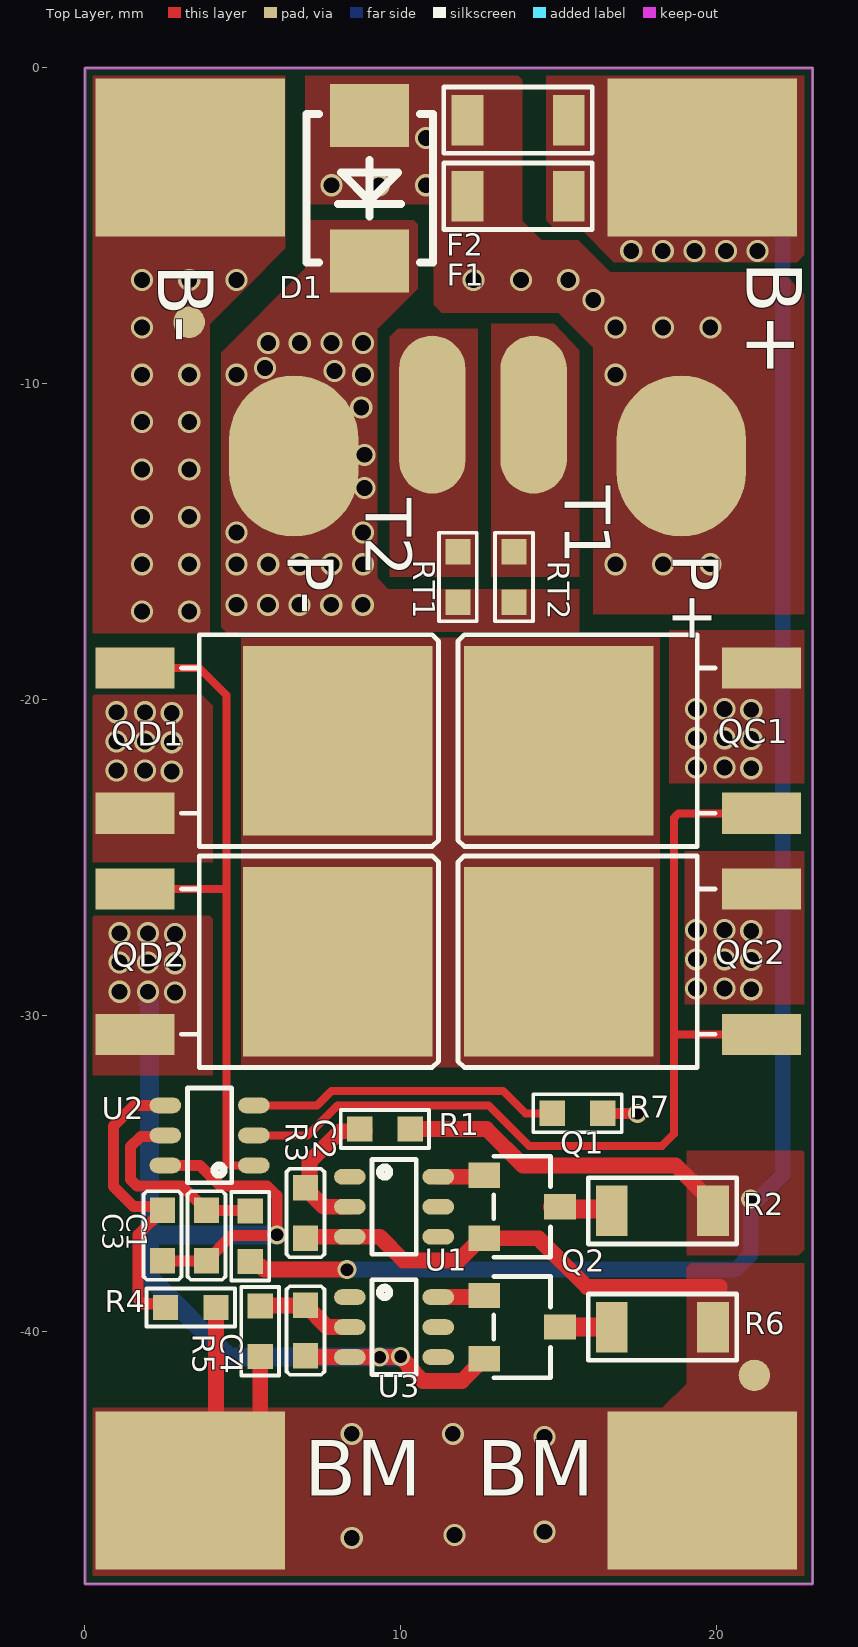
[diagram p0: Top Layer view]
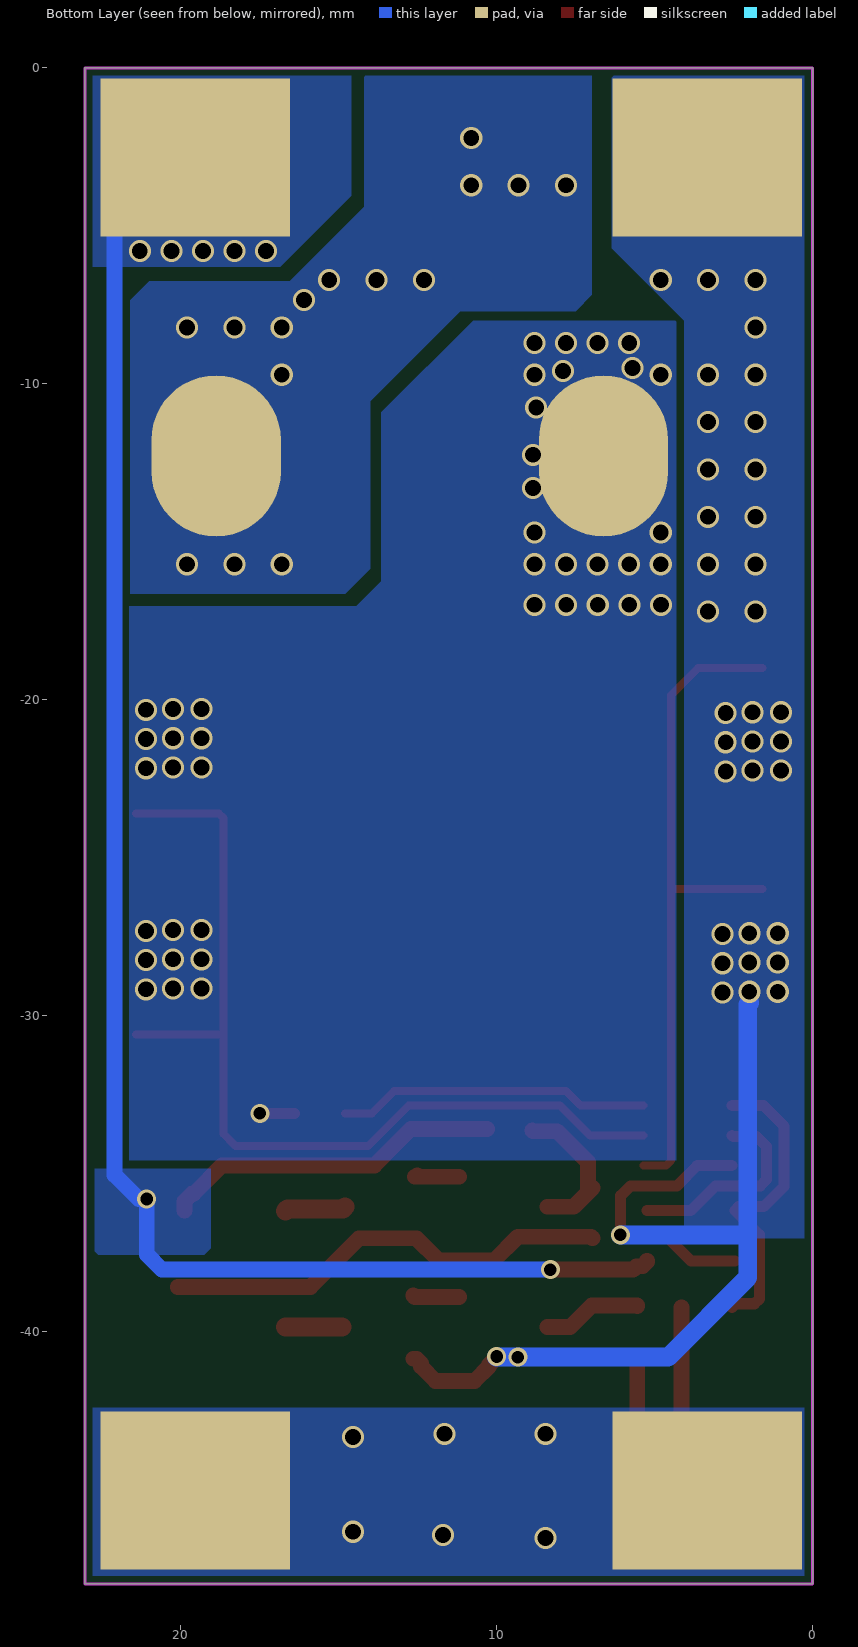
[diagram p1: Bottom Layer view, seen from below]
# Altium PCB MISC82045.PcbDoc
Units mm, origin at the board's own origin, x right, y up, seen from the top; angles counter-clockwise.
Board outline 23.04 x 48 mm, 2 copper layers (Top Layer, Bottom Layer); 33 components, 19 nets, 84 pads, 107 vias.

## Layer stack, top to bottom (the 12.6 mil dielectric is the usual default, probably not edited)
Top Solder: solder mask 0.0102, Solder Resist, Dk 3.5
Top Layer: signal copper 0.0356
Dielectric 1: dielectric 0.32, FR-4, Dk 4.8
Bottom Layer: signal copper 0.0356
Bottom Solder: solder mask 0.0102, Solder Resist, Dk 3.5

## Board outline
0,-48 23.039,-48 23.039,0 0,0

## Design rules (kind name [scope] priority, off if disabled: settings)
Clearance [All] p1: gap=0.2 ignorepadtopadclearanceinfootprint=FALSE
PolygonConnect [All] p1: connectstyle=Direct reliefconductorwidth=0.254 reliefentries=4 polygonreliefangle="90 Angle" airgapwidth=0.254
RoutingVias [All] p1: holewidth=0.711 width=1.27 viastyle="Through Hole" minholewidth=0.711 minwidth=1.27 maxholewidth=0.711 maxwidth=1.27
SilkToSilkClearance [All] p1: silktosilkclearance=0
SilkToSolderMaskClearance [IsPad] p1: minsilkscreentomaskgap=0 clearancetoexposedcopper=TRUE
SolderMaskExpansion [All] p1: expansion=0.102 istentingtop=FALSE
SupplyNets "Schematic Supply Nets" [InNet('P-')] p1: voltage=0.000
Width [All] p1: maxlimit=100 minlimit=0.254 preferedwidth=0.254
28 further rules are at their usual default settings.

## Components (designator, comment, footprint, x,y, rotation, side; value= is the part's Value field where it differs from the comment)
B+ "Pad" Pad10X8mm#1 19.546,-2.84 r90 top locked
B- "Pad" Pad10X8mm#2 4.156,-3.902 r90 top locked
BM "Pad" Pad10X8mm#1 19.546,-45.04 r90 top
BM "Pad" Pad10X8mm#1 3.338,-45.04 r270 top
C1 "0.1uF" C0603A 3.85,-36.971 r90 top
C2 "0.1uF" C0603A 6.983,-36.259 r90 top
C3 "0.1uF" C0603A 2.46,-36.971 r90 top
C4 "0.1uF" C0603A 6.985,-39.978 r90 top
D1 "RS2M" "SMB A (1+2-)" 9.017,-3.81 r90 top
F1 "F12F10 32V10A" R1206A 13.716,-4.064 r180 top
F2 "F12F10 32V10A" R1206A 13.716,-1.651 r180 top
P+ "Pad" Pad10X8mm#3 18.883,-12.286 r0 top
P- "Pad" Pad10X8mm#3 6.618,-12.286 r180 top
Q1 "3400" SOT23-3L 13.843,-36.06 r270 top
Q2 "3400" SOT23-3L 13.843,-39.87 r270 top
QC1 "N MOS*" TO-252 18.213,-21.3 r90 top
QC2 "N MOS*" TO-252 18.213,-28.3 r90 top
QD1 "N MOS*" TO-252 4.8,-21.3 r270 top
QD2 "N MOS*" TO-252 4.8,-28.3 r270 top
R1 "1K" R0603A 9.5,-33.6 r0 top
R2 "100R" R1206A 18.288,-36.187 r0 top
R3 "470R" R0603A 5.237,-36.996 r90 top
R4 "470R" R0603A 3.35,-39.25 r180 top
R5 "1K" R0603A 5.55,-40 r270 top
R6 "100R" R1206A 18.288,-39.87 r0 top
R7 "2K" R0603A 15.6,-33.1 r180 top
RT1 "NC" R0603A 11.811,-16.118 r90 top
RT2 "NC" R0603A 13.589,-16.118 r90 top
T1 "Pad" Pad10X8mm#4 14.208,-10.977 r180 top
T2 "Pad" Pad10X8mm#4 10.998,-10.977 r180 top
U1 "CM1010" SOT23-6A 9.79,-36.06 r0 top
U2 "S-8252*" SOT23-6A 3.95,-33.8 r180 top
U3 "CM1010" SOT23-6A 9.79,-39.87 r0 top

## Footprints (in the part's own frame and the unit in brackets; to place one, negate y for a bottom-side part, rotate by r counter-clockwise, add the part's x,y. Pads: shape width x height; smd on the part's side, far side on the other; paste and mask are expansions set on the pad)
C0603A [mm] "贴片电容"
  rect 0.8x0.8 smd mask+0.08: 1(-0.8,0) 2(0.8,0)
  silkscreen extent -1.4,-0.6 1.4,0.6
Pad10X8mm#1 [mm]
  rect 5x6 smd: 1(0,0)
Pad10X8mm#2 [mm]
  rect 5x6 smd: 1(1.062,0.818)
Pad10X8mm#3 [mm]
  oval 4.1x5.1 smd: 1(0,0)
Pad10X8mm#4 [mm]
  oval 2.1x5 smd: 1(0,0)
R0603A [mm] "贴片电阻"
  rect 0.8x0.8 smd mask+0.08: 1(-0.8,0) 2(0.8,0)
  silkscreen extent -1.4,-0.6 1.4,0.6
R1206A [mm] "贴片电阻"
  rect 1x1.6 smd: 1(-1.6,0) 2(1.6,0)
  silkscreen extent -2.35,-1.05 2.35,1.05
"SMB A (1+2-)" [mm] "贴片二极管"
  rect 2x2.5 smd: 1(2.3,0) 2(-2.3,0)
  silkscreen extent -2.35,-2 2.35,2
SOT23-3L [mm] "贴片IMOS"
  rect 0.8x1 smd: 1(-1,-1.2) 2(1,-1.2) 3(0,1.2)
  silkscreen extent -1.6,-0.9 1.6,0.9
SOT23-6A [mm]
  oval 1x0.5 smd mask+0.05: 1(-1.4,0.95) 2(-1.4,0) 3(-1.4,-0.95) 4(1.4,-0.95) 5(1.4,0) 6(1.4,0.95)
  silkscreen extent -0.7,-1.5 0.7,1.5
TO-252 [mm]
  rect 1.3x2.5 smd: 1(-2.3,-3.212) 2(2.3,-3.212)
  rect 6x6 smd: 3(0,3.213)
  silkscreen extent -3.35,-1.75 3.35,6.4

## Part data
B+ B- BM BM P+ P- T1 T2: "Connection pad (non-through-hole)"
C1 C2 C3 C4: library part CAP, "SMD capacitor"
D1: "SMD diode"
F1 F2: library part FUSE
Q1 Q2: library part "N MOS*", "SMD MOSFET"
QC1 QC2 QD1 QD2: "SMD MOSFET"
R1 R2 R3 R4 R5 R6 R7 RT1 RT2: library part RES, "SMD resistor"
U1 U3: "Chuangxinwei, balancing IC"
U2: library part S-8252, "2S battery protection IC"

## Free pads (board coordinates)
  rect 6x5 smd far side: 620(3.338,-45.04) 620(3.338,-2.84) 620(19.546,-45.04) 620(19.546,-2.84)
  oval 4.1x5.1 smd far side: 621(6.618,-12.286) 621(18.883,-12.286)
  round 1 smd: 622(3.3,-8.05) 622(21.2,-41.4)

## Via types
v1: diameter 0.7, hole 0.5, Top Layer to Bottom Layer, tented both sides, 101 vias
v2: diameter 0.6, hole 0.4, Top Layer to Bottom Layer, tented both sides, 6 vias

## Nets (pads, with @x,y where several pads share a name; then routed paths per layer and width w, separated by ;. In a path a pad name is that pad's centre, name@x,y a point inside that pad or via, vN(x,y) a via of type N, cw(c..) or ccw(c..) an arc to the next point about the centre after c; other vN are vias at no path point)
B+: B+.1 F1.1 F2.1 pad.620@19.546,-2.84 R1.2 R2.2 R3.1 | length 63.5
  Top Layer w0.5: R3.1@5.239,-37.771 5.239,-37.798 5.387,-37.946 5.576,-37.946 5.68,-38.05 v2(8.3,-38.05) ; R1.2 12.719,-33.6 13.869,-34.75 18.7,-34.75 19.587,-35.637 19.638,-35.637 19.888,-35.887 R2.2
  Bottom Layer w0.5: v2(8.3,-38.05) 20.6,-38.05 21.082,-37.568 v2(21.082,-35.814) 21.336,-35.814 22.1,-35.05 22.1,-5.09 19.85,-2.84 pad.620@19.546,-2.84
  other v1: 17.3,-5.8 18.3,-5.8 19.3,-5.8 20.3,-5.8 21.3,-5.8
B-: B-.1 C1.1 C3.1 C4.1 pad.620@3.338,-2.84 pad.622@3.3,-8.05 Q2.2 QD1.2 QD2.2 U2.6 U3.3 | length 37.4
  Top Layer w0.35: C3.1 C1.1 4.65,-36.971 6.135,-36.971 v2@6.198,-36.908 ; U2.6 3.65,-34.75 4.296,-35.396 5.767,-35.396 6.083,-35.712 v2(6.083,-36.95)
  Top Layer w0.5: C4.1 7.027,-40.82 U3.3 v2(9.332,-40.82) v2@10.02,-40.82 ; v2@10.019,-40.821 10.019,-40.846 10.24,-41.067 10.24,-41.11 10.704,-41.574 11.939,-41.574 12.393,-41.12 12.393,-41.02 12.543,-40.87 Q2.2
  Bottom Layer w0.6: v1@2,-29.6 2.05,-29.65 2.05,-36.95 ; v2(6.083,-36.95) 2.05,-36.95 ; v2@10,-40.82 4.57,-40.82 2.05,-38.3 2.05,-36.95
  other v1: 2.85,-29.275 1.1,-29.25 2,-29.25 2.85,-28.35 1.1,-28.325 2,-28.325 2.85,-27.425 1.1,-27.4 2,-27.4 2.75,-22.275 1,-22.25 1.9,-22.25 2.75,-21.35 1,-21.325 1.9,-21.325 2.75,-20.425 1,-20.4 1.9,-20.4 1.805,-17.214 3.305,-17.214 1.805,-15.714 3.305,-15.714 1.805,-14.214 3.305,-14.214 1.805,-12.714 3.305,-12.714 1.805,-11.214 3.305,-11.214 1.805,-9.714 3.305,-9.714 1.805,-8.214 1.805,-6.714 3.305,-6.714 4.805,-6.714
  other v2: 10,-40.8
BM: BM.1 C2.1 pad.620@3.338,-45.04 pad.620@19.546,-45.04 pad.622@21.2,-41.4 Q1.2 R4.1 R5.2 R6.2 U1.3 | length 27.4
  Top Layer w0.35: BM.1@1.443,-43.145 BM.1@3.338,-45.04
  Top Layer w0.5: BM.1@3.338,-45.04 BM.1@5.55,-42.828 ; BM.1@4.15,-44.328 R4.1 ; BM.1@5.55,-42.928 R5.2 ; C2.1@6.963,-37.059 7.012,-37.01 U1.3 9.332,-37.01 10.086,-37.764 11.839,-37.764 12.543,-37.06 Q1.2 14.36,-37.06 15.9,-38.6 20.1,-38.6
  other v1: 8.45,-46.55 11.7,-46.45 14.55,-46.35 14.55,-43.35 8.45,-43.25 11.65,-43.25
CO: QC1.1 QC2.1 U2.2 | length 30
  Top Layer w0.254: U2.2 7.05,-33.8 8,-32.85 12.785,-32.85 14.068,-34.132 18.268,-34.132 18.65,-33.75 18.65,-30.6 ; QC2.1 18.65,-30.6 ; QC1.1 18.799,-23.6 18.65,-23.749 18.65,-30.6
DO: QD1.1 QD2.1 U2.1 | length 21.8
  Top Layer w0.254: QD2.1 4.483,-26 ; QD1.1 3.62,-19 4.483,-19.864 4.483,-26 ; U2.1 4.632,-34.75 4.483,-34.601 4.483,-26
NetC1_2: C1.2 R3.2 U2.5 | length 6.5
  Top Layer w0.35: U2.5 2.521,-33.829 1.771,-33.829 1.45,-34.15 1.45,-35.191 1.655,-35.396 3.075,-35.396 C1.2 R3.2@5.239,-36.171
NetC2_2: C2.2 R1.1 U1.2 | length 4.7
  Top Layer w0.5: C2.2@6.963,-35.459 7.564,-36.06 U1.2 ; C2.2@7.113,-35.459 7.113,-34.637 8.08,-33.67 8.852,-33.67 R1.1@8.875,-33.647
NetC3_2: C3.2 R4.2 U2.4 | length 9.8
  Top Layer w0.35: R4.2 2.43,-39.13 1.83,-39.13 1.685,-38.985 1.685,-36.946 C3.2 2.343,-36.054 1.535,-36.054 0.9,-35.419 0.9,-33.505 1.555,-32.85 U2.4
NetC4_2: C4.2 R5.1 U3.2 | length 3.1
  Top Layer w0.5: R5.1 5.561,-39.189 6.974,-39.189 C4.2 7.677,-39.87 U3.2
NetQ1_1: Q1.1 U1.6 | length 1.5
  Top Layer w0.5: U1.6 Q1.1@12.593,-35.11 ; Q1.1@12.466,-35.11 Q1.1@12.516,-35.06
NetQ1_3: Q1.3 R2.1 | length 1.9
  Top Layer w0.6: Q1.3@14.8,-36.06 14.864,-36.123 16.625,-36.123 R2.1
NetQ2_1: Q2.1 U3.6 | length 1.5
  Top Layer w0.5: U3.6 12.593,-38.92 Q2.1
NetQ2_3: Q2.3 R6.1 | length 1.8
  Top Layer w0.6: Q2.3@14.9,-39.87 R6.1
NetQC1_3: QC1.3 QC2.3 QD1.3 QD2.3
NetR7_2: R7.2 U2.3 | length 9.9
  Top Layer w0.254: U2.3 7.35,-32.85 7.804,-32.396 13.246,-32.396 13.95,-33.1 R7.2
P+: D1.1 F1.2 F2.2 P+.1 pad.621@18.883,-12.286
  other v1: 16.805,-15.714 18.305,-15.714 19.805,-15.714 16.805,-9.714 16.805,-8.214 18.305,-8.214 19.805,-8.214 16.1,-7.35 12.305,-6.714 13.805,-6.714 15.305,-6.714 7.805,-3.714 9.305,-3.714 10.805,-3.714 10.805,-2.214
P-: D1.2 P-.1 pad.621@6.618,-12.286 QC1.2 QC2.2 R7.1 RT1.1 RT2.1 | length 1.1
  Top Layer w0.35: R7.1 v2(17.5,-33.1)
  other v1: 21.1,-29.175 19.35,-29.15 20.25,-29.15 21.1,-28.25 19.35,-28.225 20.25,-28.225 21.1,-27.325 19.35,-27.3 20.25,-27.3 21.1,-22.175 19.35,-22.15 20.25,-22.15 21.1,-21.25 19.35,-21.225 20.25,-21.225 21.1,-20.325 19.35,-20.3 20.25,-20.3 4.8,-17 5.8,-17 6.8,-17 7.8,-17 8.8,-17 4.805,-15.714 5.805,-15.714 6.805,-15.714 7.805,-15.714 8.805,-15.714 4.805,-14.714 8.805,-14.714 8.85,-13.3 8.85,-12.25 8.75,-10.75 4.805,-9.714 8.805,-9.714 7.9,-9.6 5.7,-9.5 5.805,-8.714 6.805,-8.714 7.805,-8.714 8.805,-8.714
T1: RT2.2 T1.1
T2: RT1.2 T2.1
pads on no net: U1.1 U1.4 U1.5 U3.1 U3.4 U3.5

## Polygon pours and split planes (outlines as drawn)
B- on Top Layer "NONET_L02_P-001" (solid, remove dead copper, pour order 19): 4.05,-25.15 4.05,-20.2 3.7,-19.85 0.3,-19.85 0.2,-19.9 0.2,-25.15
B- on Top Layer "NONET_L02_P-001" (solid, remove dead copper, pour order 18): 4.05,-31.9 4.05,-26.95 3.95,-26.85 0.3,-26.85 0.2,-26.9 0.2,-31.9
P- on Top Layer "NONET_L02_P-001" (solid, remove dead copper, pour order 17): 18.5,-22.65 23.1,-22.65 23,-22.55 23,-17.95 22.85,-17.8 18.5,-17.8
P- on Top Layer "NONET_L02_P-001" (solid, remove dead copper, pour order 16): 19,-29.65 23.1,-29.65 23,-29.55 23,-24.95 22.85,-24.8 19,-24.8
B- on Top Layer "NONET_L02_P-001" (solid, remove dead copper, pour order 2): 0,-17.65 0.25,-17.9 3.9,-17.9 3.95,-17.95 3.95,-8.115 5.08,-6.985 6.35,-5.715 6.35,-0.127 6.223,0 0,0
B+ on Top Layer "NONET_L02_P-001" (solid, remove dead copper, pour order 11): 19.05,-34.29 19.05,-37.592 22.606,-37.592 23.114,-37.084 23.114,-34.671 22.733,-34.29
B+ on Top Layer "NONET_L02_P-001" (solid, remove dead copper, pour order 10): 14.605,0 14.605,-4.826 14.893,-5.114 15.714,-5.114 16.75,-6.15 22.552,-6.15 23.114,-5.588 23.114,-0.075 23.039,0 14.478,0
T1 on Top Layer "NONET_L02_P-001" (solid, remove dead copper, pour order 9): 12.862,-16.118 15.656,-16.118 15.656,-8.944 14.857,-8.093 12.862,-8.093
T2 on Top Layer "NONET_L02_P-001" (solid, remove dead copper, pour order 8): 9.652,-16.118 12.446,-16.118 12.446,-8.255 9.906,-8.255 9.652,-8.509
P+ on Top Layer "NONET_L02_P-001" (solid, remove dead copper, pour order 7): 16.1,-17.3 22.987,-17.3 22.987,-11.239 22.987,-7.366 22.098,-6.477 16.637,-6.477 15.621,-5.461 14.461,-5.461 13.843,-4.843 13.843,-0.381 13.462,0 6.985,0 6.985,-4.318 11.049,-4.318 11.049,-7.493 11.303,-7.747 14.986,-7.747 16.1,-8.861
P- on Top Layer "NONET_L02_P-001" (solid, remove dead copper, pour order 6): 4.318,-17.718 4.65,-18.05 15.656,-18.05 15.656,-16.5 9.6,-16.5 9.25,-16.15 9.25,-8.276 10.541,-6.985 10.541,-4.953 10.414,-4.826 6.985,-4.826 6.985,-6.35 4.318,-9.017
NetQC1_3 on Top Layer "NONET_L02_P-001" (solid, remove dead copper, pour order 3): 4.95,-18.05 4.95,-31.65 18.2,-31.65 18.2,-18.05
BM on Top Layer "NONET_L02_P-001" (solid, remove dead copper, pour order 0): 18.288,-42.418 19.05,-41.656 19.05,-37.973 19.177,-37.846 23.039,-37.846 23.039,-48 0,-48 0.127,-47.873 0.127,-42.545 0.254,-42.418
P+ on Bottom Layer "NONET_L02_P-001" (solid, remove dead copper, pour order 15): 6.985,0 6.985,-7.185 7.5,-7.7 11.15,-7.7 14,-10.55 14,-15.85 14.8,-16.65 21.6,-16.65 21.6,-7.35 21,-6.75 16.55,-6.75 14.2,-4.4 14.2,-0.3 13.9,0
B+ on Bottom Layer "NONET_L02_P-001" (solid, remove dead copper, pour order 14): 23.039,-6.261 23,-6.3 16.85,-6.3 14.605,-4.055 14.605,0 23.039,0
P- on Bottom Layer "NONET_L02_P-001" (solid, remove dead copper, pour order 13): 13.65,-16.25 13.65,-10.9 10.75,-8 4.318,-8 4.318,-34.585 21.7,-34.585 21.7,-17.05 14.45,-17.05
B+ on Bottom Layer "NONET_L02_P-001" (solid, remove dead copper, pour order 12): 19.05,-34.85 19.05,-37.378 19.259,-37.587 22.611,-37.587 22.733,-37.465 22.733,-34.85
B- on Bottom Layer "NONET_L02_P-001" (solid, remove dead copper, pour order 5): 0,-37.05 4.064,-37.05 4.064,-8.001 6.35,-5.715 6.35,-0.31 6.04,0 0,0
BM on Bottom Layer "NONET_L02_P-001" (solid, remove dead copper, pour order 1): 0.127,-42.545 0.127,-47.873 0,-48 23.039,-48 23.039,-42.47 22.987,-42.418 0.254,-42.418 0.19,-42.481

## Keep-outs
Keep-Out Layer:
  the board outline again, w0.1